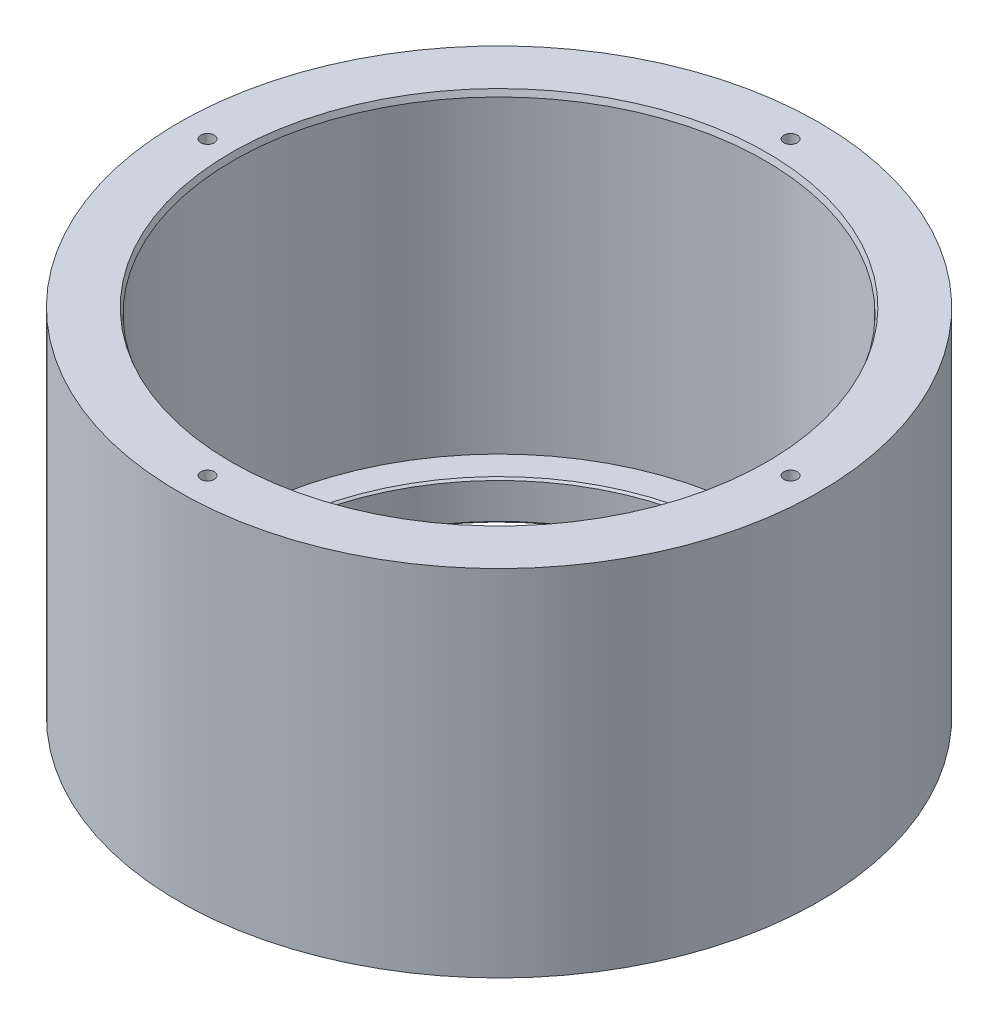
SolidWorks part; units mm, degrees
material "Q235B"
ref_plane "Front Plane" through (0, 0, 0) normal (0, 0, 1) x (1, 0, 0)
ref_plane "Top Plane" through (0, 0, 0) normal (0, 1, 0) x (1, 0, 0)
ref_plane "Right Plane" through (0, 0, 0) normal (1, 0, 0) x (0, 0, -1)
sketch "Sketch1" plane through (0, 0, 0) normal (0, 1, 0) x (1, 0, 0)
  circle A0 centre (0, 0) radius 120
  circle A1 centre (0, 0) radius 162.5
  dimension "D1" = 240
  dimension "D2" = 325
extrude "Boss-Extrude1" add sketch "Sketch1" along normal blind 180
sketch "Sketch2" plane through (0, 180, 0) normal (0, 1, 0) x (1, 0, 0)
  circle A0 centre (0, 0) radius 135
  dimension "D1" = 270
extrude "Cut-Extrude1" cut sketch "Sketch2" against normal blind 160
chamfer "Chamfer1" distance 1 distance2 3 1 edges at (0, 180, 135)
chamfer "Chamfer2" distance 1 angle 45 2 edges at (0, 20, 120) (0, 0, 120)
hole_wizard "M8 Tapped Hole1" positions "Sketch3" profile "Sketch4" tap size "M8" standard "GB"
sketch "Sketch3" plane through (0, 180, 0) normal (0, 1, 0) x (1, 0, 0)
  circle A0 centre (0, 0) radius 148
  point P0 (148, 0)
  point P11 (0, -148)
  point P12 (-148, 0)
  point P13 (0, 148)
  dimension "D1" = 296
  dimension "D2" = 4
sketch "Sketch4" plane through (148, 180, 0) normal (1, 0, 0) x (0, 0, 1)
  line L0 (0, 0) -> (0, 28.0429)
  line L1 (0, 28.0429) -> (3.4, 26)
  line L2 (3.4, 26) -> (3.4, 0)
  line L5 (3.4, 0) -> (0, 0)
  line L10 (0, 28.0429) -> (-3.4, 26) construction
  line L11 (0, -6.35) -> (0, 107.95) construction
  dimension "螺纹孔钻头直径" = 6.8
  dimension "螺纹孔钻头深度" = 26
  dimension "导头角度" = 118
cosmetic thread "Hole Cosmetic Thread1" parameters "D1"=20, "D2"=8
cosmetic thread "Hole Cosmetic Thread2" parameters "D1"=20, "D2"=8
cosmetic thread "Hole Cosmetic Thread3" parameters "D1"=20, "D2"=8
cosmetic thread "Hole Cosmetic Thread4" parameters "D1"=20, "D2"=8
